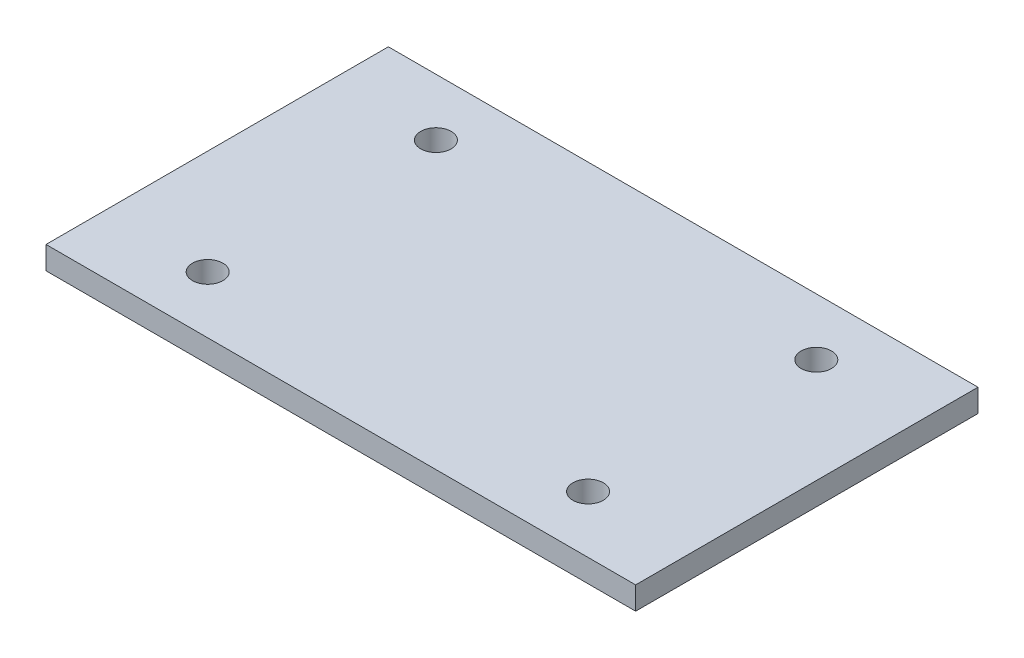
from build123d import *

# Parameters (mm, degrees)
SKETCH1_W      = 310
SKETCH1_H      = 180
SKETCH1_R      = 8
EXTRUDE1_DEPTH = 6


with BuildPart() as part:
    # Sketch1 → Extrude1 (new, symmetric)
    with BuildSketch(Plane(origin=(0, 0, 0), x_dir=(1, 0, 0), z_dir=(0, 1, 0))):
        Rectangle(SKETCH1_W, SKETCH1_H)
        with Locations(Location((100, -60, 0), (0, 0, 270))):
            Circle(SKETCH1_R, mode=Mode.SUBTRACT)
        with Locations(Location((-100, -60, 0), (0, 0, 270))):
            Circle(SKETCH1_R, mode=Mode.SUBTRACT)
        with Locations(Location((-100, 60, 0), (0, 0, 270))):
            Circle(SKETCH1_R, mode=Mode.SUBTRACT)
        with Locations(Location((100, 60, 0), (0, 0, 270))):
            Circle(SKETCH1_R, mode=Mode.SUBTRACT)
    extrude(amount=EXTRUDE1_DEPTH, both=True)


solid = part.part
